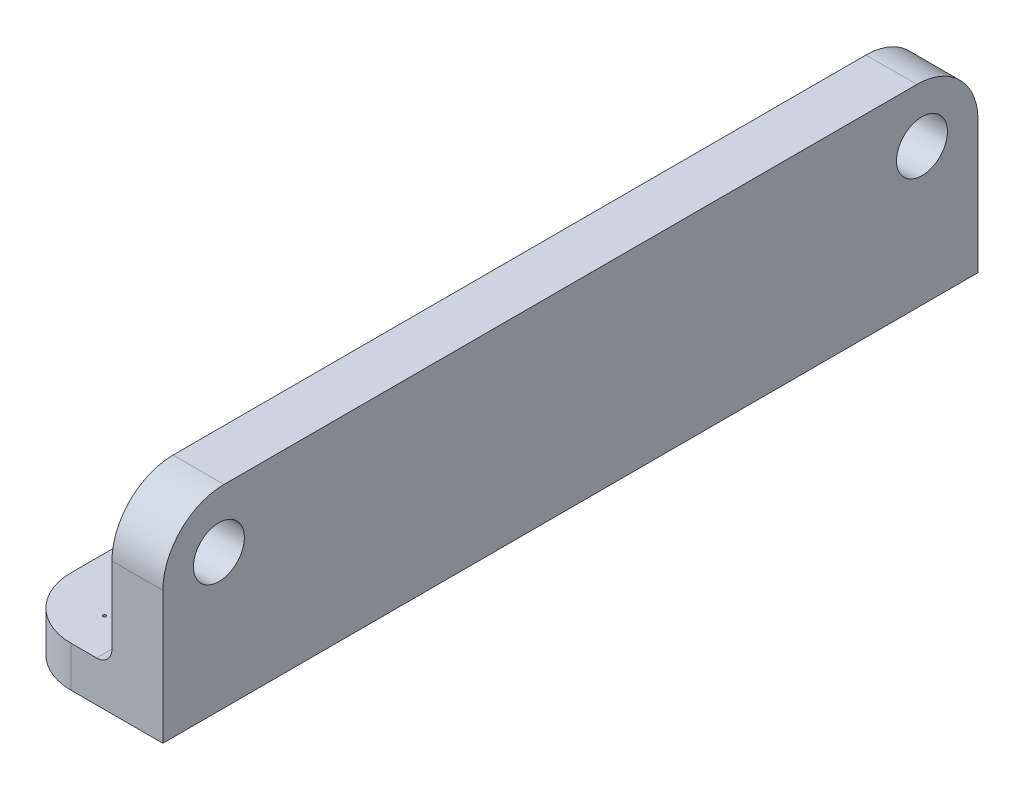
from build123d import *

# Parameters (mm, degrees)
BOSS_EXTRUDE1_DEPTH = 160
SKETCH2_R           = 5
CUT_EXTRUDE1_DEPTH  = 10
FILLET1_R           = 12
SKETCH3_R           = 0.29
CUT_EXTRUDE2_DEPTH  = 10
FILLET2_R           = 12
CUT_EXTRUDE3_DEPTH  = 2


with BuildPart() as part:
    # Sketch1 → Boss-Extrude1 (new body)
    with BuildSketch(Plane.XY):
        with BuildLine():
            Line((0, 0), (0, 38))
            Line((0, 38), (-10, 38))
            Line((-10, 38), (-10, 11))
            ThreePointArc((-10, 11), (-10.878679656, 8.878679656), (-13, 8))
            Line((-13, 8), (-30, 8))
            Line((-30, 8), (-30, 0))
            Line((-30, 0), (0, 0))
        make_face()
    extrude(amount=BOSS_EXTRUDE1_DEPTH)

    # Sketch2 → Cut-Extrude1 (cut)
    with BuildSketch(Plane(origin=(0, 0, 0), x_dir=(0, 0, -1), z_dir=(1, 0, 0))):
        with Locations((-149, 27)):
            Circle(SKETCH2_R)
        with Locations((-11, 27)):
            Circle(SKETCH2_R)
    extrude(amount=-CUT_EXTRUDE1_DEPTH, mode=Mode.SUBTRACT)

    # Fillet1
    fillet1_edges = [part.edges().sort_by_distance(p)[0] for p in [
        (-5, 38, 160),
        (-5, 38, 0),
    ]]
    fillet(fillet1_edges, radius=FILLET1_R)

    # Sketch3 → Cut-Extrude2 (cut)
    with BuildSketch(Plane.XZ):
        with Locations(Location((-19.4, 152.04, 0), (0, 0, 270))):
            Circle(SKETCH3_R)
        with Locations(Location((-19.4, 132.04, 0), (0, 0, 270))):
            Circle(SKETCH3_R)
        with Locations(Location((-19.4, 112.04, 0), (0, 0, 270))):
            Circle(SKETCH3_R)
        with Locations(Location((-19.4, 92.04, 0), (0, 0, 270))):
            Circle(SKETCH3_R)
        with Locations(Location((-19.4, 72.04, 0), (0, 0, 270))):
            Circle(SKETCH3_R)
        with Locations(Location((-19.4, 52.04, 0), (0, 0, 270))):
            Circle(SKETCH3_R)
        with Locations(Location((-19.4, 32.04, 0), (0, 0, 270))):
            Circle(SKETCH3_R)
        with Locations(Location((-19.4, 12.04, 0), (0, 0, 270))):
            Circle(SKETCH3_R)
    extrude(amount=-CUT_EXTRUDE2_DEPTH, mode=Mode.SUBTRACT)

    # Fillet2
    fillet2_edges = [part.edges().sort_by_distance(p)[0] for p in [
        (-30, 4, 160),
        (-30, 4, 0),
    ]]
    fillet(fillet2_edges, radius=FILLET2_R)

    # Sketch4 → Cut-Extrude3 (cut)
    # profile 1 of 14: a face of its own
    with BuildSketch(Plane.ZY.offset(10)):
        with BuildLine():
            add(Edge.make_bspline(
                [(43.789463141, 27.128205128), (43.885401956, 27.125990241), (44.073971614, 27.121636835), (44.350602112, 27.084519537), (44.614775522, 27.025139559), (44.866102187, 26.94032377), (45.104751783, 26.83164906), (45.331100809, 26.698906573), (45.544477107, 26.541694182), (45.742271885, 26.362027206), (45.921943943, 26.166315593), (46.081171888, 25.959435655), (46.213392756, 25.740471418), (46.323922783, 25.512591424), (46.407556672, 25.273681613), (46.469520423, 25.025766171), (46.506065098, 24.767184246), (46.5105467, 24.591260773), (46.512820513, 24.502003205)],
                knots=[0, 0, 0, 0, 1.090651108, 2.14369656, 3.167927427, 4.165692988, 5.154576575, 6.145033357, 7.14440862, 8.163220312, 9.178978109, 10.162394332, 11.12677451, 12.082874982, 13.037579715, 13.999894772, 14.985214855, 16, 16, 16, 16], degree=3))
            add(Edge.make_bspline(
                [(46.512820513, 24.502003205), (46.51059042, 24.413402109), (46.506195327, 24.238786063), (46.468948479, 23.981779842), (46.408900448, 23.734164805), (46.324807686, 23.495458754), (46.214493884, 23.267482456), (46.081611731, 23.048323208), (45.923341765, 22.84007439), (45.744340167, 22.642992783), (45.547629507, 22.462680769), (45.336414412, 22.304326422), (45.113256925, 22.171042552), (44.879268747, 22.060089835), (44.632535755, 21.976789826), (44.374900226, 21.915019383), (44.105348031, 21.878523769), (43.92178503, 21.874061787), (43.828525641, 21.871794872)],
                knots=[0, 0, 0, 0, 1.015667565, 2.001689161, 2.971180881, 3.933912672, 4.898051938, 5.870540525, 6.8683264, 7.892867857, 8.919988739, 9.923897136, 10.914753654, 11.896185405, 12.887840524, 13.895451133, 14.930781579, 16, 16, 16, 16], degree=3))
            add(Edge.make_bspline(
                [(43.828525641, 21.871794872), (43.737584021, 21.873993245), (43.558637985, 21.878318988), (43.296121281, 21.91578961), (43.044258463, 21.974203705), (42.803374952, 22.058155846), (42.573088135, 22.165235279), (42.354710017, 22.298064805), (42.14631105, 22.452770383), (41.951855251, 22.629999269), (41.774387936, 22.824075404), (41.618722114, 23.030662067), (41.486327455, 23.247131224), (41.378626719, 23.473730472), (41.294724398, 23.71067502), (41.236520667, 23.957907915), (41.198841052, 24.214724483), (41.194506876, 24.389355866), (41.192307692, 24.477964744)],
                knots=[0, 0, 0, 0, 1.056734814, 2.079339537, 3.076314658, 4.058285941, 5.039336339, 6.023146808, 7.024524339, 8.052147497, 9.076900738, 10.077495695, 11.054668894, 12.021676166, 12.988994953, 13.970866516, 14.970407042, 16, 16, 16, 16], degree=3))
            add(Edge.make_bspline(
                [(41.192307692, 24.477964744), (41.193070754, 24.537440259), (41.194587252, 24.65564098), (41.212871443, 24.831160665), (41.239349386, 25.003876706), (41.277495711, 25.173207847), (41.326698397, 25.339184222), (41.387342842, 25.501457135), (41.456802648, 25.661398116), (41.539651559, 25.815832357), (41.629602274, 25.96565673), (41.729557079, 26.106847244), (41.835287134, 26.241123158), (41.951244052, 26.364899994), (42.073550805, 26.481806442), (42.204206291, 26.590038566), (42.342409318, 26.690574299), (42.488755624, 26.781174762), (42.63963886, 26.86311639), (42.795177118, 26.933433318), (42.953257933, 26.993784835), (43.114621716, 27.042700299), (43.278839962, 27.081317493), (43.446271083, 27.107613713), (43.616781692, 27.125934167), (43.731655005, 27.127444884), (43.789463141, 27.128205128)],
                knots=[0, 0, 0, 0, 1.036913812, 2.060746492, 3.074578145, 4.08324605, 5.085523353, 6.091481477, 7.103103322, 8.124200051, 9.145827961, 10.149052085, 11.139400635, 12.124186929, 13.104469564, 14.088618662, 15.081002312, 16.082788945, 17.088477375, 18.073521874, 19.057670972, 20.037642247, 21.012252997, 21.997331918, 22.992189685, 24, 24, 24, 24], degree=3))
        make_face()
        with BuildLine():
            add(Edge.make_bspline(
                [(43.810496795, 26.551282051), (43.768392233, 26.550615557), (43.684645321, 26.549289885), (43.559884775, 26.535413503), (43.436416145, 26.514569173), (43.314025572, 26.485253849), (43.192612149, 26.448623742), (43.073220902, 26.401763555), (42.954698267, 26.348147409), (42.839158371, 26.284592136), (42.726526253, 26.215603036), (42.619992796, 26.138585871), (42.518335324, 26.056719764), (42.423018791, 25.967246647), (42.334222146, 25.8713379), (42.251452285, 25.769151274), (42.174077461, 25.661040207), (42.103792059, 25.546255336), (42.038875585, 25.427172316), (41.984230557, 25.303020221), (41.937942168, 25.175120007), (41.899951801, 25.043606338), (41.869513823, 24.908219047), (41.849149122, 24.768907943), (41.835228743, 24.625817045), (41.83397159, 24.529080893), (41.833333333, 24.479967949)],
                knots=[0, 0, 0, 0, 0.951425037, 1.892405618, 2.834142553, 3.780555396, 4.735506122, 5.698386817, 6.677778342, 7.674036042, 8.677244726, 9.661625187, 10.643485342, 11.625954439, 12.613944774, 13.595804929, 14.596853729, 15.616869823, 16.636634596, 17.660413109, 18.67984269, 19.709280547, 20.753005387, 21.813969624, 22.890152378, 24, 24, 24, 24], degree=3))
            add(Edge.make_bspline(
                [(41.833333333, 24.479967949), (41.834883752, 24.408418164), (41.83792468, 24.268083377), (41.867251478, 24.06223947), (41.912718102, 23.865540705), (41.977073993, 23.67818616), (42.059939038, 23.500232527), (42.161359562, 23.331731213), (42.28150558, 23.172259987), (42.41894373, 23.02488331), (42.56794045, 22.890221956), (42.725981533, 22.772879579), (42.889448702, 22.671411063), (43.060965335, 22.590080936), (43.238850237, 22.526699088), (43.423405396, 22.481598503), (43.614664901, 22.453713395), (43.744629801, 22.45039814), (43.810496795, 22.448717949)],
                knots=[0, 0, 0, 0, 1.087324682, 2.132633634, 3.154656843, 4.153212625, 5.138884617, 6.133989092, 7.13811672, 8.169089965, 9.193543553, 10.187520856, 11.158295186, 12.114249704, 13.068004623, 14.02467326, 14.998892505, 16, 16, 16, 16], degree=3))
            add(Edge.make_bspline(
                [(43.810496795, 22.448717949), (43.857270389, 22.449386199), (43.950002138, 22.45071105), (44.087466708, 22.464393853), (44.222211358, 22.485490906), (44.354315478, 22.513891061), (44.483385771, 22.553060565), (44.61039624, 22.598122565), (44.733952741, 22.654319682), (44.854942878, 22.716489936), (44.970277892, 22.78798893), (45.081257575, 22.863997292), (45.185639215, 22.946700665), (45.281420784, 23.037752512), (45.372507102, 23.13302819), (45.456425823, 23.235200968), (45.533763803, 23.343603813), (45.603745328, 23.457889591), (45.666516178, 23.576689326), (45.722308592, 23.699121906), (45.767656182, 23.825367935), (45.806569046, 23.954192562), (45.835259783, 24.086910526), (45.85600539, 24.222718844), (45.869855004, 24.361827432), (45.871142979, 24.455562132), (45.871794872, 24.503004808)],
                knots=[0, 0, 0, 0, 1.036970321, 2.055862331, 3.060095599, 4.060719653, 5.049301004, 6.049377071, 7.046955997, 8.056986028, 9.063944937, 10.053856218, 11.039021426, 12.013303897, 12.982198174, 13.960523328, 14.942567566, 15.933032457, 16.929951754, 17.920776327, 18.913894254, 19.902475604, 20.903099658, 21.921964767, 22.948227815, 24, 24, 24, 24], degree=3))
            add(Edge.make_bspline(
                [(45.871794872, 24.503004808), (45.871139992, 24.550113535), (45.869846209, 24.643181691), (45.856074966, 24.780966519), (45.835284089, 24.915112771), (45.806391635, 25.046107093), (45.767853178, 25.173375568), (45.722272232, 25.297892257), (45.666513363, 25.418332481), (45.603706898, 25.535110393), (45.533589324, 25.647879114), (45.455354164, 25.754523201), (45.371151327, 25.856276049), (45.27973364, 25.95163833), (45.181040812, 26.04095755), (45.076010094, 26.124902702), (44.964325347, 26.203797288), (44.845710483, 26.274847113), (44.723332925, 26.340129952), (44.597843679, 26.395802412), (44.47141309, 26.44452681), (44.342875416, 26.483670095), (44.212255004, 26.513515855), (44.079876175, 26.535782997), (43.945658381, 26.549168361), (43.855598536, 26.550576739), (43.810496795, 26.551282051)],
                knots=[0, 0, 0, 0, 1.048789873, 2.071992723, 3.080474812, 4.070813472, 5.056451928, 6.039816187, 7.021295338, 8.009314668, 8.991328769, 9.975844821, 10.952581135, 11.930703152, 12.91499457, 13.914777939, 14.923479275, 15.957618598, 16.991998452, 18.010408503, 19.012925223, 20.00783076, 20.999814803, 21.994803685, 22.995802798, 24, 24, 24, 24], degree=3))
        make_face(mode=Mode.SUBTRACT)
    # profile 2 of 14: a face of its own
    with BuildSketch(Plane.ZY.offset(10)):
        Polygon((47.538461538, 27), (48.179487179, 27), (48.179487179, 22.576923077), (50.038461538, 22.576923077), (50.038461538, 22), (47.538461538, 22), align=None)
    # profile 3 of 14: a face of its own
    with BuildSketch(Plane.ZY.offset(10)):
        with BuildLine():
            Line((50.807692308, 22), (50.807692308, 27))
            Line((50.807692308, 27), (51.866386218, 27))
            add(Edge.make_bspline(
                [(51.866386218, 27), (51.955535039, 26.99937861), (52.127192906, 26.998182111), (52.375350039, 26.990335505), (52.604207015, 26.976843125), (52.814254227, 26.956505855), (53.005280648, 26.932587437), (53.177225581, 26.900943795), (53.330746192, 26.866832105), (53.424752377, 26.835462074), (53.468950321, 26.820713141)],
                knots=[0, 0, 0, 0, 1.321377177, 2.544338591, 3.679698859, 4.71869479, 5.671952218, 6.531967125, 7.309789724, 8, 8, 8, 8], degree=3))
            add(Edge.make_bspline(
                [(53.468950321, 26.820713141), (53.530832293, 26.797395244), (53.652971198, 26.751371785), (53.826025512, 26.664979821), (53.989520145, 26.570198615), (54.14141801, 26.462610613), (54.281429042, 26.342893569), (54.411956055, 26.213662272), (54.528971623, 26.071148895), (54.636158501, 25.919375495), (54.731130534, 25.758166551), (54.81333706, 25.58963956), (54.882767455, 25.414118123), (54.939868236, 25.232049043), (54.983629553, 25.043104569), (55.015966847, 24.847798739), (55.035289141, 24.645626184), (55.037395199, 24.50838847), (55.038461538, 24.438902244)],
                knots=[0, 0, 0, 0, 1.037989101, 2.048720264, 3.03347809, 4.003905725, 4.967380877, 5.923996735, 6.884742632, 7.859453364, 8.839691521, 9.819957728, 10.801471334, 11.80152298, 12.813966534, 13.844978706, 14.908869198, 16, 16, 16, 16], degree=3))
            add(Edge.make_bspline(
                [(55.038461538, 24.438902244), (55.037529943, 24.378773296), (55.03568966, 24.259993919), (55.020122771, 24.084077485), (54.995486707, 23.913098211), (54.960272021, 23.747165711), (54.915245747, 23.586514876), (54.859773621, 23.430694539), (54.795106054, 23.279506077), (54.719713927, 23.13467166), (54.637072423, 22.996626591), (54.546721611, 22.867359134), (54.450461629, 22.746825824), (54.348071084, 22.635014637), (54.238597779, 22.532517903), (54.12218527, 22.439414024), (53.999521727, 22.354750165), (53.869421059, 22.279110461), (53.729452051, 22.21186064), (53.577034684, 22.155416084), (53.411867528, 22.10767171), (53.234115825, 22.067078028), (53.042845816, 22.038179017), (52.839004508, 22.016307106), (52.622476678, 22.001585313), (52.473716399, 22.000538295), (52.397235577, 22)],
                knots=[0, 0, 0, 0, 1.058131973, 2.090245403, 3.105765157, 4.096918797, 5.07359586, 6.040054961, 7.006085223, 7.965371986, 8.911666288, 9.835956746, 10.738988486, 11.624821356, 12.502036588, 13.375701924, 14.24610047, 15.122941669, 16.021834204, 16.975760622, 17.979893693, 19.046217526, 20.182340398, 21.382202726, 22.654134781, 24, 24, 24, 24], degree=3))
            Line((52.397235577, 22), (50.807692308, 22))
        make_face()
        with BuildLine():
            Line((51.448717949, 22.576923077), (51.883413462, 22.576923077))
            add(Edge.make_bspline(
                [(51.883413462, 22.576923077), (51.963547965, 22.577231716), (52.117497617, 22.577824655), (52.338858058, 22.584397248), (52.541002033, 22.592244793), (52.723281071, 22.606815095), (52.886094562, 22.623076015), (53.029445896, 22.64408718), (53.153921143, 22.667715035), (53.229033392, 22.689902909), (53.263621795, 22.700120192)],
                knots=[0, 0, 0, 0, 1.383618687, 2.658126108, 3.823786659, 4.876093986, 5.815132222, 6.648351516, 7.377580062, 8, 8, 8, 8], degree=3))
            add(Edge.make_bspline(
                [(53.263621795, 22.700120192), (53.306616059, 22.715491464), (53.391543556, 22.745854669), (53.513234342, 22.802355795), (53.627923776, 22.867530145), (53.735227221, 22.941964811), (53.836051033, 23.02468108), (53.930475446, 23.115585406), (54.016821403, 23.216546972), (54.095622619, 23.325558518), (54.167025098, 23.441877576), (54.22908532, 23.565123383), (54.281579252, 23.695046405), (54.32302022, 23.83133255), (54.356511426, 23.973808756), (54.380342353, 24.122734399), (54.394407069, 24.278374526), (54.396414779, 24.384119083), (54.397435897, 24.437900641)],
                knots=[0, 0, 0, 0, 0.982760408, 1.941267819, 2.884666843, 3.819923004, 4.749609063, 5.690155114, 6.638335438, 7.60609908, 8.583824457, 9.574050268, 10.573936541, 11.597196452, 12.638231748, 13.723193679, 14.842018967, 16, 16, 16, 16], degree=3))
            add(Edge.make_bspline(
                [(54.397435897, 24.437900641), (54.396631121, 24.494370938), (54.39504675, 24.6055445), (54.377851728, 24.769014223), (54.353819472, 24.926534528), (54.317623593, 25.077638859), (54.269929489, 25.221858533), (54.214584583, 25.360826394), (54.146669787, 25.492401093), (54.069859208, 25.617434365), (53.984045599, 25.734622876), (53.889192082, 25.84217728), (53.78704861, 25.941241644), (53.675140622, 26.028828176), (53.556642473, 26.109110582), (53.429118015, 26.177577819), (53.293958844, 26.23768942), (53.199484351, 26.268956086), (53.151442308, 26.284855769)],
                knots=[0, 0, 0, 0, 1.129217777, 2.223100788, 3.284889252, 4.31516385, 5.326848226, 6.321524555, 7.304244934, 8.284784113, 9.254596696, 10.205833222, 11.15055266, 12.096616828, 13.045035565, 14.010353181, 14.988227444, 16, 16, 16, 16], degree=3))
            add(Edge.make_bspline(
                [(53.151442308, 26.284855769), (53.110828901, 26.29602765), (53.024557832, 26.31975898), (52.883942762, 26.347160219), (52.725490437, 26.370649253), (52.548468096, 26.390780738), (52.35368072, 26.405471323), (52.140220742, 26.414675878), (51.908842298, 26.422408539), (51.748204671, 26.422848971), (51.665064103, 26.423076923)],
                knots=[0, 0, 0, 0, 0.675026783, 1.433893058, 2.294494921, 3.24250292, 4.28921909, 5.425097092, 6.667317884, 8, 8, 8, 8], degree=3))
            Line((51.665064103, 26.423076923), (51.448717949, 26.423076923))
            Line((51.448717949, 26.423076923), (51.448717949, 22.576923077))
        make_face(mode=Mode.SUBTRACT)
    # profile 4 of 14: a face of its own
    with BuildSketch(Plane.ZY.offset(10)):
        Polygon((62.057692308, 27), (64.397435897, 22), (63.739383013, 22), (62.980168269, 23.602564103), (60.934895833, 23.602564103), (60.17568109, 22), (59.525641026, 22), (61.857371795, 27), align=None)
        Polygon((61.957532051, 25.907251603), (61.179286859, 24.179487179), (62.743790064, 24.179487179), align=None, mode=Mode.SUBTRACT)
    # profile 5 of 14: a face of its own
    with BuildSketch(Plane.ZY.offset(10)):
        Polygon((64.846153846, 22), (65.514222756, 27), (65.766626603, 27), (67.662660256, 23.025641026), (69.55869391, 27), (69.815104167, 27), (70.487179487, 22), (69.851161859, 22), (69.406450321, 25.525641026), (67.783854167, 22), (67.541466346, 22), (65.923878205, 25.525641026), (65.481169872, 22), align=None)
    # profile 6 of 14: a face of its own
    with BuildSketch(Plane.ZY.offset(10)):
        Polygon((73.467948718, 27), (75.807692308, 22), (75.149639423, 22), (74.390424679, 23.602564103), (72.345152244, 23.602564103), (71.5859375, 22), (70.935897436, 22), (73.267628205, 27), align=None)
        Polygon((73.367788462, 25.907251603), (72.589543269, 24.179487179), (74.154046474, 24.179487179), align=None, mode=Mode.SUBTRACT)
    # profile 7 of 14: a face of its own
    with BuildSketch(Plane.ZY.offset(10)):
        Polygon((76.512820513, 27), (77.153846154, 27), (77.153846154, 22.576923077), (79.012820513, 22.576923077), (79.012820513, 22), (76.512820513, 22), align=None)
    # profile 8 of 14: a face of its own
    with BuildSketch(Plane.ZY.offset(10)):
        with BuildLine():
            Line((84.525641026, 26.140625), (84.039863782, 25.717948718))
            add(Edge.make_bspline(
                [(84.039863782, 25.717948718), (83.963651982, 25.784496998), (83.815287533, 25.9140491), (83.582980152, 26.085180935), (83.349372888, 26.229525953), (83.114403887, 26.345360964), (82.882039345, 26.43813722), (82.651220427, 26.501920573), (82.423782439, 26.543591203), (82.272541371, 26.548741041), (82.197916667, 26.551282051)],
                knots=[0, 0, 0, 0, 1.174203348, 2.285866929, 3.345479548, 4.357773815, 5.323690501, 6.245291137, 7.134199255, 8, 8, 8, 8], degree=3))
            add(Edge.make_bspline(
                [(82.197916667, 26.551282051), (82.154811759, 26.550606825), (82.068736719, 26.549258483), (81.940315196, 26.535393584), (81.813145804, 26.514711513), (81.687151124, 26.485111948), (81.562064606, 26.44861599), (81.438843737, 26.402075364), (81.316730311, 26.347635147), (81.196714035, 26.284984706), (81.080063071, 26.215484898), (80.969194637, 26.13899676), (80.864799937, 26.055644489), (80.766683339, 25.965663916), (80.675421068, 25.868917699), (80.589660667, 25.766797645), (80.511623311, 25.656909857), (80.439789923, 25.541620762), (80.37644286, 25.421749146), (80.31942597, 25.300179573), (80.272487878, 25.175881055), (80.234501105, 25.049267417), (80.204245654, 24.920504254), (80.182282515, 24.789733412), (80.168691225, 24.656539844), (80.167345575, 24.567139584), (80.166666667, 24.522035256)],
                knots=[0, 0, 0, 0, 0.9732313, 1.943419598, 2.914105962, 3.881741322, 4.864768402, 5.855028487, 6.854206409, 7.882911434, 8.911035887, 9.919250175, 10.922630637, 11.925982763, 12.923451909, 13.924676513, 14.935397504, 15.964931351, 16.990480746, 17.995899336, 18.995873688, 19.988284801, 20.979664002, 21.981342857, 22.981544644, 24, 24, 24, 24], degree=3))
            add(Edge.make_bspline(
                [(80.166666667, 24.522035256), (80.167814907, 24.475937934), (80.170107437, 24.383901902), (80.182835196, 24.246901395), (80.206136746, 24.112419635), (80.238504077, 23.980305039), (80.2793973, 23.850395268), (80.329550246, 23.722355756), (80.390308135, 23.597469583), (80.457687504, 23.4745893), (80.533510344, 23.356655675), (80.617236306, 23.245493452), (80.70603872, 23.139666759), (80.802583188, 23.042121677), (80.903959634, 22.949594415), (81.013702379, 22.866152746), (81.128727818, 22.787695277), (81.249802118, 22.716620868), (81.3758537, 22.653939106), (81.504792953, 22.598633484), (81.637041119, 22.552395768), (81.771781454, 22.51428429), (81.90972077, 22.485303732), (82.049858155, 22.464507058), (82.192964923, 22.450660587), (82.289363711, 22.44937065), (82.338141026, 22.448717949)],
                knots=[0, 0, 0, 0, 0.993588149, 1.983757546, 2.962012758, 3.932297264, 4.913089422, 5.895147596, 6.892791648, 7.904042674, 8.913936126, 9.911190904, 10.901569418, 11.888649192, 12.866825019, 13.856968273, 14.856789458, 15.866221433, 16.879824684, 17.888846278, 18.887838639, 19.896937192, 20.90452114, 21.923117541, 22.949107649, 24, 24, 24, 24], degree=3))
            add(Edge.make_bspline(
                [(82.338141026, 22.448717949), (82.398965518, 22.450086761), (82.518944118, 22.452786793), (82.69505452, 22.473461899), (82.864405068, 22.505384742), (83.025270227, 22.555000169), (83.180215058, 22.614013463), (83.326928128, 22.689190191), (83.467166152, 22.776354719), (83.597915665, 22.877486067), (83.719766708, 22.986411015), (83.828279559, 23.103675251), (83.925322366, 23.225474173), (84.007140275, 23.354732851), (84.078159992, 23.487828441), (84.134417041, 23.62756704), (84.178024928, 23.772761185), (84.196059611, 23.87278218), (84.205128205, 23.923076923)],
                knots=[0, 0, 0, 0, 1.125101743, 2.219305524, 3.276925285, 4.308813505, 5.329771737, 6.340890082, 7.353855978, 8.380572537, 9.395307413, 10.374367262, 11.333343716, 12.272376171, 13.200803521, 14.12078735, 15.055053215, 16, 16, 16, 16], degree=3))
            Line((84.205128205, 23.923076923), (82.602564103, 23.923076923))
            Line((82.602564103, 23.923076923), (82.602564103, 24.5))
            Line((82.602564103, 24.5), (84.846153846, 24.5))
            add(Edge.make_bspline(
                [(84.846153846, 24.5), (84.843881711, 24.401060213), (84.839446247, 24.20791864), (84.803837828, 23.92638263), (84.751334943, 23.66014998), (84.674629108, 23.410343761), (84.577437867, 23.176611911), (84.458733865, 22.958948878), (84.31875031, 22.757418084), (84.158431458, 22.573155949), (83.980195661, 22.407875224), (83.785933214, 22.263132432), (83.574773198, 22.143000227), (83.349412575, 22.043199148), (83.108603636, 21.966087284), (82.852966412, 21.911469581), (82.582101566, 21.877681617), (82.396335332, 21.873790225), (82.301081731, 21.871794872)],
                knots=[0, 0, 0, 0, 1.147910205, 2.240849596, 3.288798376, 4.293882934, 5.268269983, 6.221997348, 7.165762291, 8.110600512, 9.051082397, 9.981847279, 10.915696266, 11.864665164, 12.837641225, 13.844673414, 14.894833504, 16, 16, 16, 16], degree=3))
            add(Edge.make_bspline(
                [(82.301081731, 21.871794872), (82.244972821, 21.872614911), (82.133983412, 21.874237037), (81.969900162, 21.885603036), (81.810020746, 21.903166911), (81.655006093, 21.929533392), (81.504018979, 21.962153705), (81.358288928, 22.003872302), (81.215832961, 22.050100079), (81.079171546, 22.107246714), (80.945393709, 22.168568525), (80.81671799, 22.239141731), (80.693026331, 22.317748976), (80.571700575, 22.401279296), (80.457403466, 22.495010387), (80.346301466, 22.59446325), (80.24010643, 22.701655155), (80.173290525, 22.777891967), (80.139623397, 22.81630609)],
                knots=[0, 0, 0, 0, 1.103516608, 2.18287355, 3.233646581, 4.265703846, 5.274262808, 6.270085734, 7.246073526, 8.217965859, 9.181570311, 10.139587173, 11.101556858, 12.063436887, 13.034641265, 14.006444858, 14.995489556, 16, 16, 16, 16], degree=3))
            add(Edge.make_bspline(
                [(80.139623397, 22.81630609), (80.090282034, 22.877149267), (79.992659267, 22.997528577), (79.869649564, 23.192520218), (79.761656246, 23.392113742), (79.675803313, 23.60050187), (79.608353629, 23.815651768), (79.559979723, 24.038154208), (79.531838361, 24.267904422), (79.527720084, 24.423468642), (79.525641026, 24.502003205)],
                knots=[0, 0, 0, 0, 1.024988564, 2.027958144, 3.013741914, 3.99376912, 4.974186348, 5.962951834, 6.97162285, 8, 8, 8, 8], degree=3))
            add(Edge.make_bspline(
                [(79.525641026, 24.502003205), (79.526389949, 24.560812784), (79.527874043, 24.677352106), (79.546282741, 24.850524742), (79.5726803, 25.02091543), (79.610819888, 25.188255035), (79.660089493, 25.352202372), (79.720654093, 25.512992867), (79.791355009, 25.671188083), (79.873966817, 25.824858947), (79.963877799, 25.973972113), (80.064924546, 26.113895231), (80.171927951, 26.247262269), (80.288634049, 26.370871506), (80.411694113, 26.4881623), (80.544675287, 26.595010268), (80.68482142, 26.694589876), (80.833336457, 26.784511762), (80.987797393, 26.865318519), (81.147876686, 26.936189281), (81.313261658, 26.994511239), (81.482800184, 27.044573161), (81.657806434, 27.080981794), (81.837367129, 27.107866521), (82.02193419, 27.125946037), (82.146791911, 27.127446369), (82.209935897, 27.128205128)],
                knots=[0, 0, 0, 0, 1.010042427, 2.001538926, 2.988977894, 3.97147212, 4.947868168, 5.928132478, 6.921817128, 7.922678872, 8.924230854, 9.911186466, 10.885946514, 11.860014231, 12.829900618, 13.804660667, 14.788293046, 15.781961137, 16.785220236, 17.781814947, 18.787040195, 19.796447094, 20.816926666, 21.855387176, 22.915410262, 24, 24, 24, 24], degree=3))
            add(Edge.make_bspline(
                [(82.209935897, 27.128205128), (82.263033397, 27.127263116), (82.368650132, 27.12538935), (82.525806143, 27.115638249), (82.680638116, 27.097692298), (82.832804717, 27.070934516), (82.983214902, 27.039727427), (83.130481147, 26.999218941), (83.275176643, 26.952007344), (83.418011997, 26.897774637), (83.559577559, 26.835589673), (83.700270507, 26.764470802), (83.839490129, 26.682645051), (83.978704563, 26.592688825), (84.117042067, 26.493346148), (84.254282457, 26.384556662), (84.392089505, 26.2678296), (84.480646945, 26.183480776), (84.525641026, 26.140625)],
                knots=[0, 0, 0, 0, 0.985310127, 1.959889608, 2.920407961, 3.875718043, 4.825872088, 5.769643135, 6.708031182, 7.649175746, 8.603380435, 9.575831151, 10.572468945, 11.59831001, 12.650450436, 13.731164539, 14.847254788, 16, 16, 16, 16], degree=3))
        make_face()
    # profile 9 of 14: a face of its own
    with BuildSketch(Plane.ZY.offset(10)):
        Polygon((87.955128205, 27), (90.294871795, 22), (89.63681891, 22), (88.877604167, 23.602564103), (86.832331731, 23.602564103), (86.073116987, 22), (85.423076923, 22), (87.754807692, 27), align=None)
        Polygon((87.854967949, 25.907251603), (87.076722756, 24.179487179), (88.641225962, 24.179487179), align=None, mode=Mode.SUBTRACT)
    # profile 10 of 14: a face of its own
    with BuildSketch(Plane.ZY.offset(10)):
        Polygon((90.743589744, 22), (91.411658654, 27), (91.6640625, 27), (93.560096154, 23.025641026), (95.456129808, 27), (95.712540064, 27), (96.384615385, 22), (95.748597756, 22), (95.303886218, 25.525641026), (93.681290064, 22), (93.438902244, 22), (91.821314103, 25.525641026), (91.378605769, 22), align=None)
    # profile 11 of 14: a face of its own
    with BuildSketch(Plane.ZY.offset(10)):
        Polygon((99.365384615, 27), (101.705128205, 22), (101.047075321, 22), (100.287860577, 23.602564103), (98.242588141, 23.602564103), (97.483373397, 22), (96.833333333, 22), (99.165064103, 27), align=None)
        Polygon((99.265224359, 25.907251603), (98.486979167, 24.179487179), (100.051482372, 24.179487179), align=None, mode=Mode.SUBTRACT)
    # profile 12 of 14: a face of its own
    with BuildSketch(Plane.ZY.offset(10)):
        Polygon((101.833333333, 26.423076923), (101.833333333, 27), (104.653846154, 27), (104.653846154, 26.423076923), (103.564102564, 26.423076923), (103.564102564, 22), (102.923076923, 22), (102.923076923, 26.423076923), align=None)
    # profile 13 of 14: a face of its own
    with BuildSketch(Plane.ZY.offset(10)):
        Polygon((105.294871795, 27), (108.243589744, 27), (108.243589744, 26.423076923), (105.935897436, 26.423076923), (105.935897436, 25.012820513), (108.243589744, 25.012820513), (108.243589744, 24.435897436), (105.935897436, 24.435897436), (105.935897436, 22.576923077), (108.243589744, 22.576923077), (108.243589744, 22), (105.294871795, 22), align=None)
    # profile 14 of 14: a face of its own
    with BuildSketch(Plane.ZY.offset(10)):
        with BuildLine():
            Line((109.076923077, 22), (109.076923077, 27))
            Line((109.076923077, 27), (110.135616987, 27))
            add(Edge.make_bspline(
                [(110.135616987, 27), (110.224765809, 26.99937861), (110.396423675, 26.998182111), (110.644580808, 26.990335505), (110.873437784, 26.976843125), (111.083484996, 26.956505855), (111.274511418, 26.932587437), (111.44645635, 26.900943795), (111.599976962, 26.866832105), (111.693983146, 26.835462074), (111.73818109, 26.820713141)],
                knots=[0, 0, 0, 0, 1.321377177, 2.544338591, 3.679698859, 4.71869479, 5.671952218, 6.531967125, 7.309789724, 8, 8, 8, 8], degree=3))
            add(Edge.make_bspline(
                [(111.73818109, 26.820713141), (111.800063063, 26.797395244), (111.922201967, 26.751371785), (112.095256281, 26.664979821), (112.258750914, 26.570198615), (112.410648779, 26.462610613), (112.550659811, 26.342893569), (112.681186825, 26.213662272), (112.798202392, 26.071148895), (112.90538927, 25.919375495), (113.000361303, 25.758166551), (113.082567829, 25.58963956), (113.151998224, 25.414118123), (113.209099005, 25.232049043), (113.252860322, 25.043104569), (113.285197616, 24.847798739), (113.304519911, 24.645626184), (113.306625968, 24.50838847), (113.307692308, 24.438902244)],
                knots=[0, 0, 0, 0, 1.037989101, 2.048720264, 3.03347809, 4.003905725, 4.967380877, 5.923996735, 6.884742632, 7.859453364, 8.839691521, 9.819957728, 10.801471334, 11.80152298, 12.813966534, 13.844978706, 14.908869198, 16, 16, 16, 16], degree=3))
            add(Edge.make_bspline(
                [(113.307692308, 24.438902244), (113.306760712, 24.378773296), (113.304920429, 24.259993919), (113.28935354, 24.084077485), (113.264717476, 23.913098211), (113.22950279, 23.747165711), (113.184476516, 23.586514876), (113.12900439, 23.430694539), (113.064336823, 23.279506077), (112.988944696, 23.13467166), (112.906303193, 22.996626591), (112.815952381, 22.867359134), (112.719692398, 22.746825824), (112.617301853, 22.635014637), (112.507828548, 22.532517903), (112.39141604, 22.439414024), (112.268752496, 22.354750165), (112.138651828, 22.279110461), (111.998682821, 22.21186064), (111.846265453, 22.155416084), (111.681098297, 22.10767171), (111.503346594, 22.067078028), (111.312076585, 22.038179017), (111.108235277, 22.016307106), (110.891707448, 22.001585313), (110.742947168, 22.000538295), (110.666466346, 22)],
                knots=[0, 0, 0, 0, 1.058131973, 2.090245403, 3.105765157, 4.096918797, 5.07359586, 6.040054961, 7.006085223, 7.965371986, 8.911666288, 9.835956746, 10.738988486, 11.624821356, 12.502036588, 13.375701924, 14.24610047, 15.122941669, 16.021834204, 16.975760622, 17.979893693, 19.046217526, 20.182340398, 21.382202726, 22.654134781, 24, 24, 24, 24], degree=3))
            Line((110.666466346, 22), (109.076923077, 22))
        make_face()
        with BuildLine():
            Line((109.717948718, 22.576923077), (110.152644231, 22.576923077))
            add(Edge.make_bspline(
                [(110.152644231, 22.576923077), (110.232778734, 22.577231716), (110.386728387, 22.577824655), (110.608088827, 22.584397248), (110.810232802, 22.592244793), (110.99251184, 22.606815095), (111.155325331, 22.623076015), (111.298676666, 22.64408718), (111.423151912, 22.667715035), (111.498264162, 22.689902909), (111.532852564, 22.700120192)],
                knots=[0, 0, 0, 0, 1.383618687, 2.658126108, 3.823786659, 4.876093986, 5.815132222, 6.648351516, 7.377580062, 8, 8, 8, 8], degree=3))
            add(Edge.make_bspline(
                [(111.532852564, 22.700120192), (111.575846828, 22.715491464), (111.660774325, 22.745854669), (111.782465111, 22.802355795), (111.897154545, 22.867530145), (112.004457991, 22.941964811), (112.105281802, 23.02468108), (112.199706215, 23.115585406), (112.286052172, 23.216546972), (112.364853388, 23.325558518), (112.436255867, 23.441877576), (112.498316089, 23.565123383), (112.550810021, 23.695046405), (112.592250989, 23.83133255), (112.625742196, 23.973808756), (112.649573122, 24.122734399), (112.663637838, 24.278374526), (112.665645548, 24.384119083), (112.666666667, 24.437900641)],
                knots=[0, 0, 0, 0, 0.982760408, 1.941267819, 2.884666843, 3.819923004, 4.749609063, 5.690155114, 6.638335438, 7.60609908, 8.583824457, 9.574050268, 10.573936541, 11.597196452, 12.638231748, 13.723193679, 14.842018967, 16, 16, 16, 16], degree=3))
            add(Edge.make_bspline(
                [(112.666666667, 24.437900641), (112.66586189, 24.494370938), (112.66427752, 24.6055445), (112.647082497, 24.769014223), (112.623050242, 24.926534528), (112.586854362, 25.077638859), (112.539160258, 25.221858533), (112.483815353, 25.360826394), (112.415900557, 25.492401093), (112.339089978, 25.617434365), (112.253276368, 25.734622876), (112.158422851, 25.84217728), (112.056279379, 25.941241644), (111.944371391, 26.028828176), (111.825873242, 26.109110582), (111.698348784, 26.177577819), (111.563189613, 26.23768942), (111.46871512, 26.268956086), (111.420673077, 26.284855769)],
                knots=[0, 0, 0, 0, 1.129217777, 2.223100788, 3.284889252, 4.31516385, 5.326848226, 6.321524555, 7.304244934, 8.284784113, 9.254596696, 10.205833222, 11.15055266, 12.096616828, 13.045035565, 14.010353181, 14.988227444, 16, 16, 16, 16], degree=3))
            add(Edge.make_bspline(
                [(111.420673077, 26.284855769), (111.38005967, 26.29602765), (111.293788601, 26.31975898), (111.153173531, 26.347160219), (110.994721207, 26.370649253), (110.817698866, 26.390780738), (110.622911489, 26.405471323), (110.409451511, 26.414675878), (110.178073067, 26.422408539), (110.017435441, 26.422848971), (109.934294872, 26.423076923)],
                knots=[0, 0, 0, 0, 0.675026783, 1.433893058, 2.294494921, 3.24250292, 4.28921909, 5.425097092, 6.667317884, 8, 8, 8, 8], degree=3))
            Line((109.934294872, 26.423076923), (109.717948718, 26.423076923))
            Line((109.717948718, 26.423076923), (109.717948718, 22.576923077))
        make_face(mode=Mode.SUBTRACT)
    extrude(amount=-CUT_EXTRUDE3_DEPTH, mode=Mode.SUBTRACT)


solid = part.part
